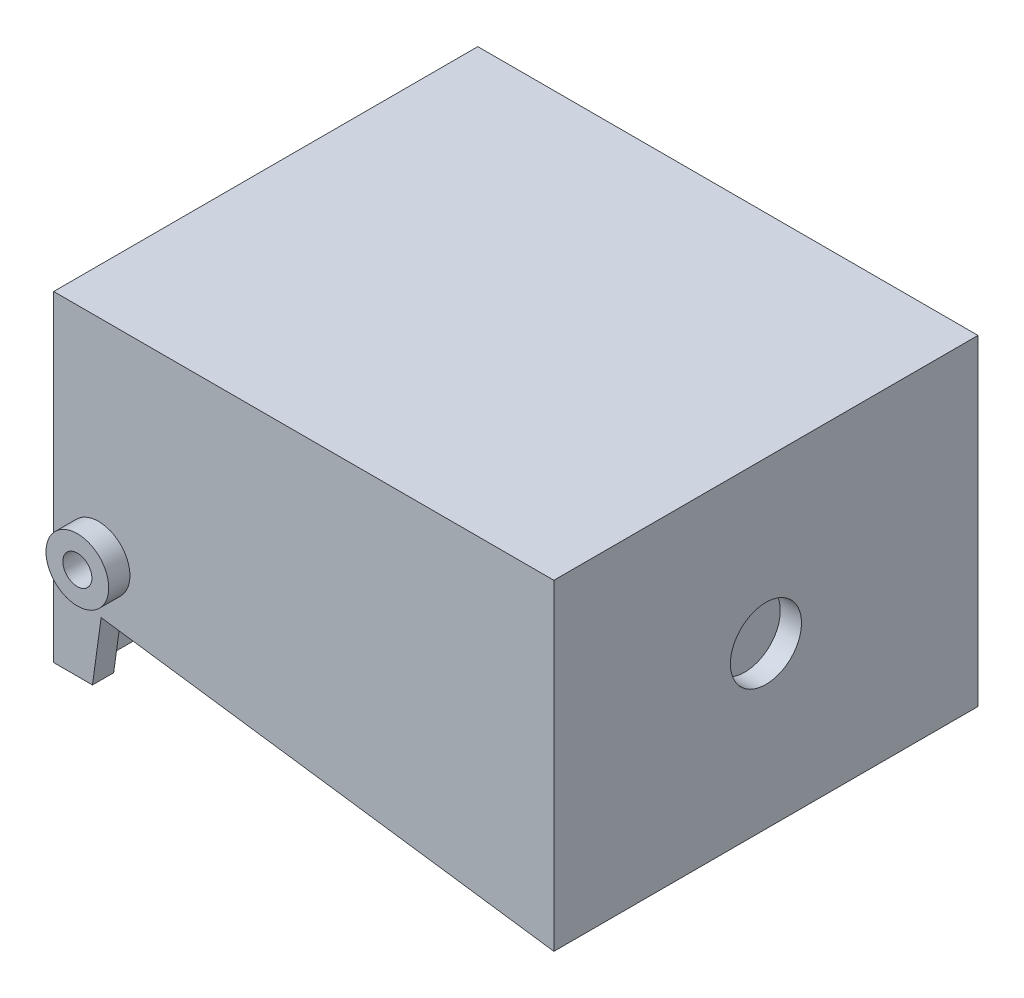
SolidWorks part; units mm, degrees
ref_plane "Front Plane" through (0, 0, 0) normal (0, 0, 1) x (1, 0, 0)
ref_plane "Top Plane" through (0, 0, 0) normal (0, 1, 0) x (1, 0, 0)
ref_plane "Right Plane" through (0, 0, 0) normal (1, 0, 0) x (0, 0, -1)
other "Configuration Table"
sketch "Sketch1" plane through (0, 0, 0) normal (0, 0, 1) x (1, 0, 0)
  line L0 (-60, 0) -> (0, 0) construction
  line L1 (-32.6139, 0) -> (-44.4075, 0)
  line L2 (-32.6139, 0) -> (-32.6139, -7.5777)
  line L3 (-32.6139, -7.5777) -> (-44.4075, -7.5777)
  line L4 (-44.4075, 0) -> (-44.4075, -7.5777)
extrude "Boss-Extrude1" add sketch "Sketch1" against normal up to surface (10 mm away)
shell "Shell1" thickness 0.5
sketch "Sketch2" plane through (0, 0, 0) normal (0, 0, 1) x (1, 0, 0)
  line L0 (-32.6139, -7.5777) -> (-43.288, -6.0987)
  line L1 (-43.288, -6.0987) -> (-43.4929, -7.5777)
  line L2 (-44.4075, -7.5777) -> (-32.6139, -7.5777) construction
  line L3 (-43.4929, -7.5777) -> (-42.3222, -12.9142)
  line L4 (-42.3222, -12.9142) -> (-34.2098, -9.4651)
  line L5 (-34.2098, -9.4651) -> (-32.6139, -7.5777)
extrude "Cut-Extrude1" cut sketch "Sketch2" against normal through all both and the other way through all
sketch "Sketch3" plane through (0, 0, 0) normal (0, 0, 1) x (1, 0, 0)
  circle A0 centre (-43.3489, -4.9039) radius 0.7394
extrude "Boss-Extrude2" add sketch "Sketch3" along normal blind 0.5
sketch "Sketch4" plane through (0, 0, 0.5) normal (0, 0, 1) x (1, 0, 0)
  circle A0 centre (-43.3489, -4.9039) radius 0.3422
extrude "Cut-Extrude2" cut sketch "Sketch4" against normal through all both and the other way through all
sketch "Sketch5" plane through (-32.6139, 0, 0) normal (1, 0, 0) x (0, 0, -1)
  circle A0 centre (5, -3.7889) radius 0.8381
extrude "Cut-Extrude3" cut sketch "Sketch5" against normal blind 0.5 and the other way through all
sketch "Sketch6" plane through (-43.9075, 0, 0) normal (1, 0, 0) x (0, 0, -1)
  circle A0 centre (5, -4.0389) radius 1.1766
extrude "Boss-Extrude3" add sketch "Sketch6" along normal blind 1.5
sketch "Sketch7" plane through (-42.4075, 0, 0) normal (1, 0, 0) x (0, 0, -1)
  circle A0 centre (5, -4.0389) radius 2
  dimension "D1" = 4
extrude "Boss-Extrude4" add sketch "Sketch7" along normal blind 3
sketch "Sketch8" plane through (-39.4075, 0, 0) normal (1, 0, 0) x (0, 0, -1)
  circle A0 centre (5, -4.0389) radius 2.5
  dimension "D1" = 5
extrude "Boss-Extrude5" add sketch "Sketch8" along normal blind 3
sketch "Sketch9" plane through (-36.4075, 0, 0) normal (1, 0, 0) x (0, 0, -1)
  circle A0 centre (5, -4.0389) radius 2.9444
extrude "Boss-Extrude6" add sketch "Sketch9" along normal up to surface (3.2936 mm away) up to face at (-33.1139, -3.7889, -5.8381)
